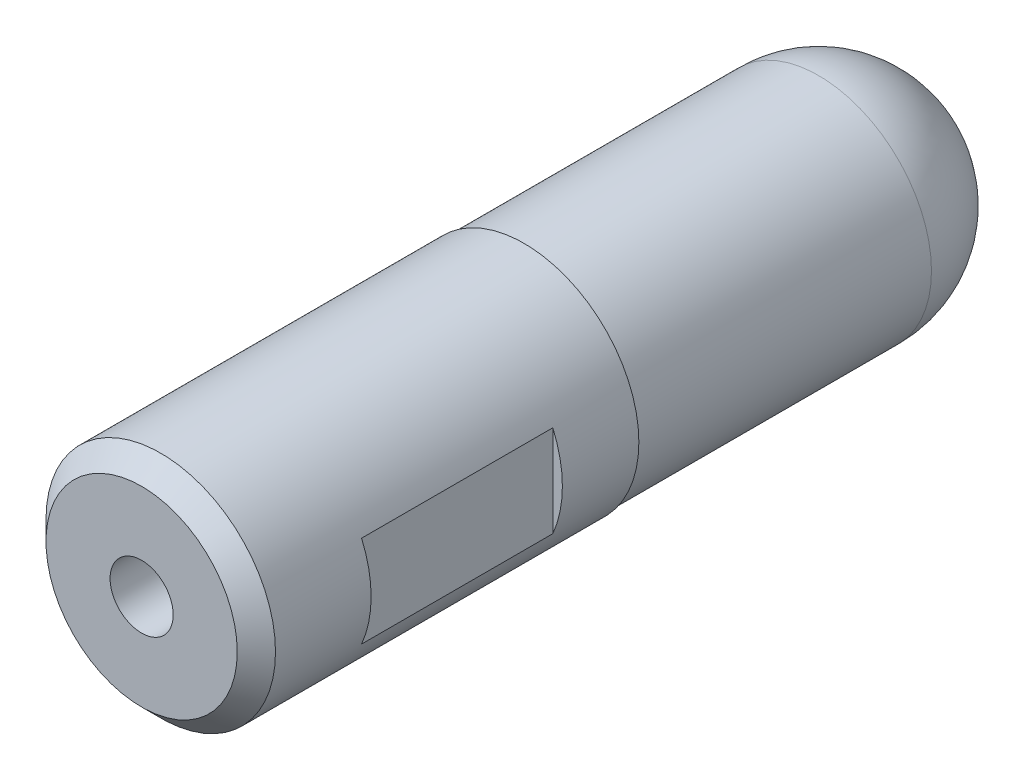
from build123d import *

# Parameters (mm, degrees)
SKETCH1_R               = 5.9
BOSS_EXTRUDE1_DEPTH     = 35.4
M4_TAPPED_HOLE1_D       = 3.3
M4_TAPPED_HOLE1_DEPTH   = 10.1
M4_TAPPED_HOLE1_TIP     = 0.991420021
SKETCH5_R               = 6
SKETCH5_R_2             = 4
BOSS_EXTRUDE2_DEPTH     = 20
CHAMFER1_SIZE           = 1
CUT_EXTRUDE1_DEPTH      = 37.402747149
CUT_EXTRUDE1_DEPTH_BACK = 37.402747149
SKETCH6_W               = 2.026292368
SKETCH6_H               = 10


with BuildPart() as part:
    # Sketch1 → Boss-Extrude1 (new body)
    with BuildSketch(Plane.XY):
        Circle(SKETCH1_R)
    extrude(amount=BOSS_EXTRUDE1_DEPTH)

    # Sketch2 → Revolve1 (revolve)
    with BuildSketch(Plane(origin=(0, 0, 0), x_dir=(1, 0, 0), z_dir=(0, 1, 0))):
        with BuildLine():
            Line((0, 5.9), (0, 0))
            Line((0, 0), (-5.9, 0))
            ThreePointArc((-5.9, 0), (-4.171930009, 4.171930009), (0, 5.9))
        make_face()
    revolve(axis=Axis((0, 0, -5.9), (0, 0, 1)))

    # M4 Tapped Hole1
    with Locations(Plane.XY.offset(35.4)):
        with Locations((0, 0)):
            Hole(M4_TAPPED_HOLE1_D / 2, depth=M4_TAPPED_HOLE1_DEPTH)
            with Locations((0, 0, -(M4_TAPPED_HOLE1_DEPTH + M4_TAPPED_HOLE1_TIP / 2))):  # 118° drill point
                Cone(0, M4_TAPPED_HOLE1_D / 2, M4_TAPPED_HOLE1_TIP, mode=Mode.SUBTRACT)

    # Sketch5 → Boss-Extrude2 (add)
    with BuildSketch(Plane.XY.offset(35.4)):
        Circle(SKETCH5_R)
        Circle(SKETCH5_R_2, mode=Mode.SUBTRACT)
    extrude(amount=-BOSS_EXTRUDE2_DEPTH)

    # Chamfer1
    chamfer1_edges = [part.edges().sort_by_distance(p)[0] for p in [
        (-6, 0, 35.4),
    ]]
    chamfer(chamfer1_edges, length=CHAMFER1_SIZE)

    # Sketch6 → Cut-Extrude1 (cut, two sides: drawn at the far end of the back side and taken through both)
    with BuildSketch(Plane(origin=(0, 0, 0), x_dir=(1, 0, 0), z_dir=(0, 1, 0)).offset(-CUT_EXTRUDE1_DEPTH_BACK)):
        with Locations((-6.513146184, -24.4)):
            Rectangle(SKETCH6_W, SKETCH6_H)
        with Locations((6.513146184, -24.4)):
            Rectangle(SKETCH6_W, SKETCH6_H)
    extrude(amount=CUT_EXTRUDE1_DEPTH + CUT_EXTRUDE1_DEPTH_BACK, mode=Mode.SUBTRACT)


solid = part.part
